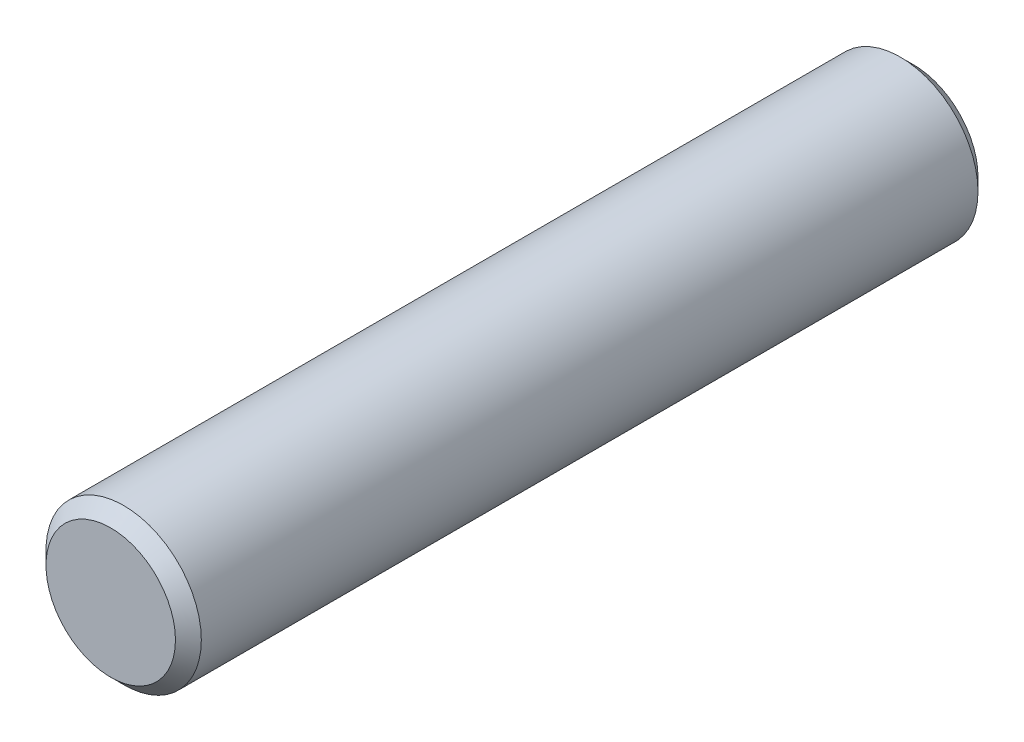
from build123d import *

# Parameters (mm, degrees)
SKETCH1_R           = 0.6
BOSS_EXTRUDE1_DEPTH = 3.1
CHAMFER1_SIZE       = 0.1


with BuildPart() as part:
    # Sketch1 → Boss-Extrude1 (new, symmetric)
    with BuildSketch(Plane.XY):
        Circle(SKETCH1_R)
    extrude(amount=BOSS_EXTRUDE1_DEPTH, both=True)

    # Chamfer1
    chamfer1_edges = [part.edges().sort_by_distance(p)[0] for p in [
        (-0.6, 0, -3.1),
        (-0.6, 0, 3.1),
    ]]
    chamfer(chamfer1_edges, length=CHAMFER1_SIZE)


solid = part.part
